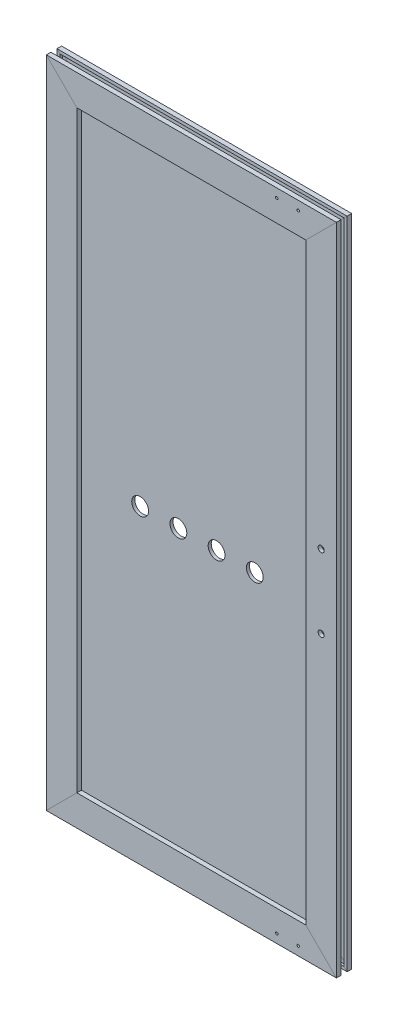
SolidWorks part; units mm, degrees
material "铝型材"
ref_plane "前视基准面" through (0, 0, 0) normal (0, 0, 1) x (1, 0, 0)
ref_plane "上视基准面" through (0, 0, 0) normal (0, 1, 0) x (1, 0, 0)
ref_plane "右视基准面" through (0, 0, 0) normal (1, 0, 0) x (0, 0, -1)
sketch "草图13" plane through (0, 0, 0) normal (0, 0, 1) x (1, 0, 0)
  line L1 (-169.75, -408) -> (169.75, -408)
  line L2 (-169.75, -408) -> (-169.75, 408)
  line L3 (-169.75, 408) -> (169.75, 408)
  line L4 (169.75, -408) -> (169.75, 408)
  line L5 (-169.75, -408) -> (169.75, 408) construction
  line L6 (-169.75, 408) -> (169.75, -408) construction
  point P0 (0, 0)
  dimension "D1" = 339.5
  dimension "D2" = 816
other "铝型材 2040A(1)"
ref_plane "基准面3" through (-169.75, 408, 0) normal (1, 0, 0) x (0, 1, 0)
sketch "草图19" plane through (-169.75, 408, 0) normal (1, 0, 0) x (0, 1, 0)
  line L0 (9, 4) -> (6, 4)
  line L1 (9, 4) -> (9, 7)
  line L2 (6, -4) -> (6, 4)
  line L3 (16, 7) -> (9, 7)
  line L4 (9, -4) -> (6, -4)
  line L5 (16, 4) -> (16, 7)
  line L6 (9, -7) -> (9, -4)
  line L7 (20, 4) -> (16, 4)
  line L8 (16, -7) -> (9, -7)
  line L9 (20, 10) -> (20, 4)
  line L10 (16, -7) -> (16, -4)
  line L11 (-20, 10) -> (20, 10)
  line L12 (20, -4) -> (16, -4)
  line L13 (-20, 4) -> (-20, 10)
  line L14 (20, -4) -> (20, -10)
  line L15 (-20, 4) -> (-16, 4)
  line L16 (20, -10) -> (-20, -10)
  line L17 (-16, 4) -> (-16, 7)
  line L18 (-20, -10) -> (-20, -4)
  line L19 (-16, 7) -> (-9, 7)
  line L20 (-20, -4) -> (-16, -4)
  line L21 (-9, 4) -> (-9, 7)
  line L22 (-16, -7) -> (-16, -4)
  line L23 (-9, 4) -> (-6, 4)
  line L24 (-16, -7) -> (-9, -7)
  line L25 (-6, -4) -> (-6, 4)
  line L26 (-9, -7) -> (-9, -4)
  line L27 (-9, -4) -> (-6, -4)
  circle A0 centre (0, 0) radius 3.25
  point P0 (0, 0)
sketch "草图14" plane through (0, 0, 0) normal (0, 0, 1) x (1, 0, 0)
  line L0 (175.75, 414) -> (178.75, 417) construction
  line L1 (-163.25, -401.5) -> (163.25, -401.5)
  line L2 (-163.25, -401.5) -> (-163.25, 401.5)
  line L3 (-163.25, 401.5) -> (163.25, 401.5)
  line L4 (163.25, -401.5) -> (163.25, 401.5)
  line L5 (-163.25, -401.5) -> (163.25, 401.5) construction
  line L6 (-163.25, 401.5) -> (163.25, -401.5) construction
  line L8 (149.75, 388) -> (-149.75, 388) construction
  point P0 (0, 0)
  dimension "D1" = 13.5
extrude "凸台-拉伸1" add sketch "草图14" along normal mid plane 4 separate body
hole_wizard "M4 螺纹孔2" positions "草图24" profile "草图25" tap size "M4" standard "GB"
sketch "草图24" plane through (0, 0, 10) normal (0, 0, -1) x (-1, 0, 0)
  line L0 (-139.75, 416.5) -> (-111.75, 416.5) construction
  line L7 (0, 0) -> (81.0682, 0) construction
  line L10 (-189.75, 428) -> (189.75, 428) construction
  line L11 (-189.75, -428) -> (-189.75, 428) construction
  point P0 (-139.75, 416.5)
  point P2 (-111.75, 416.5)
  point P29 (-111.75, -416.5)
  point P30 (-139.75, -416.5)
  dimension "D1" = 28
  dimension "D2" = 11.5
  dimension "D3" = 50
cosmetic thread "孔螺蚊线3"
cosmetic thread "孔螺蚊线4"
cosmetic thread "孔螺蚊线9"
cosmetic thread "孔螺蚊线10"
sketch "草图25" plane through (139.75, 416.5, 10) normal (1, 0, 0) x (0, -1, 0)
  line L0 (0, 0) -> (0, 11.0914)
  line L1 (0, 11.0914) -> (1.65, 10.1)
  line L2 (1.65, 10.1) -> (1.65, 0)
  line L5 (1.65, 0) -> (0, 0)
  line L10 (0, 11.0914) -> (-1.65, 10.1) construction
  line L11 (0, -6.35) -> (0, 107.95) construction
  dimension "螺纹孔钻头直径" = 3.3
  dimension "螺纹孔钻头深度" = 10.1
  dimension "导头角度" = 118
hole_wizard "打孔尺寸(%根据)开槽圆柱头螺钉的类型1" positions "草图26" profile "草图27" counterbore size "M4" standard "GB" end condition through all
sketch "草图26" plane through (0, 0, 10) normal (0, 0, 1) x (1, 0, 0)
  line L0 (0, 0) -> (50000, 0) construction
  line L1 (169.75, 424) -> (169.75, -49576) construction
  line L2 (189.75, 428) -> (149.75, 388) construction
  point P0 (169.75, 48)
  point P2 (169.75, -48)
  point P14 (169.75, 408)
  dimension "D1" = 96
sketch "草图27" plane through (169.75, 48, 10) normal (1, 0, 0) x (0, -1, 0)
  line L0 (0, 0) -> (0, 20)
  line L1 (0, 20) -> (2.25, 20)
  line L3 (2.25, 20) -> (2.25, 4.6)
  line L4 (2.25, 4.6) -> (4, 4.6)
  line L5 (4, 4.6) -> (4, 0)
  line L7 (4, 0) -> (0, 0)
  line L11 (0, -6.35) -> (0, 107.95) construction
  dimension "通孔孔直径" = 4.5
  dimension "通孔孔深度" = 20
  dimension "柱形沉头孔直径" = 8
  dimension "柱形沉头孔深度" = 4.6
hole_wizard "M6 螺纹孔1" positions "草图28" profile "草图29" tap size "M6" standard "GB"
sketch "草图28" plane through (0, 0, -10) normal (0, 0, -1) x (-1, 0, 0)
  line L0 (0, 0) -> (50000, 0) construction
  line L1 (169.75, 424) -> (169.75, -49576) construction
  line L2 (149.75, 388) -> (189.75, 428) construction
  line L3 (-189.75, 428) -> (189.75, 428) construction
  line L4 (169.75, -469.5) -> (169.75, 49530.5) construction
  point P0 (169.75, 328)
  point P2 (169.75, 291)
  point P12 (169.75, 408)
  point P19 (169.75, -328)
  point P20 (169.75, -291)
  dimension "D1" = 100
  dimension "D2" = 37
sketch "草图29" plane through (-169.75, 328, -10) normal (1, 0, 0) x (0, 1, 0)
  line L0 (0, 0) -> (0, 18.5022)
  line L1 (0, 18.5022) -> (2.5, 17)
  line L2 (2.5, 17) -> (2.5, 0)
  line L5 (2.5, 0) -> (0, 0)
  line L10 (0, 18.5022) -> (-2.5, 17) construction
  line L11 (0, -6.35) -> (0, 107.95) construction
  dimension "螺纹孔钻头直径" = 5
  dimension "螺纹孔钻头深度" = 17
  dimension "导头角度" = 118
cosmetic thread "孔螺蚊线5"
cosmetic thread "孔螺蚊线6"
cosmetic thread "孔螺蚊线7"
cosmetic thread "孔螺蚊线8"
sketch "草图30" plane through (0, 0, -2) normal (0, 0, -1) x (-1, 0, 0)
  line L0 (0, 0) -> (0, 30) construction
  line L1 (100, 30) -> (-100, 30)
  line L2 (100, 30) -> (100, 170)
  line L3 (100, 170) -> (-100, 170)
  line L4 (-100, 30) -> (-100, 170)
  line L5 (100, 30) -> (-100, 170) construction
  line L6 (100, 170) -> (-100, 30) construction
  point P0 (0, 100)
  dimension "D1" = 200
  dimension "D2" = 140
  dimension "D3" = 30
extrude "凸台-拉伸2" add sketch "草图30" along normal blind 5 separate body
sketch "草图31" plane through (0, 0, -2) normal (0, 0, -1) x (-1, 0, 0)
  line L0 (-75, -30) -> (-25, -30) construction
  line L1 (-25, -30) -> (25, -30) construction
  line L2 (25, -30) -> (75, -30) construction
  line L3 (0, -30) -> (0, 0) construction
  circle A0 centre (-75, -30) radius 11
  circle A1 centre (-25, -30) radius 11
  circle A2 centre (25, -30) radius 11
  circle A3 centre (75, -30) radius 11
  dimension "D1" = 22
  dimension "D2" = 50
  dimension "D3" = 30
extrude "切除-拉伸1" cut sketch "草图31" against normal up to next (4 mm away)
